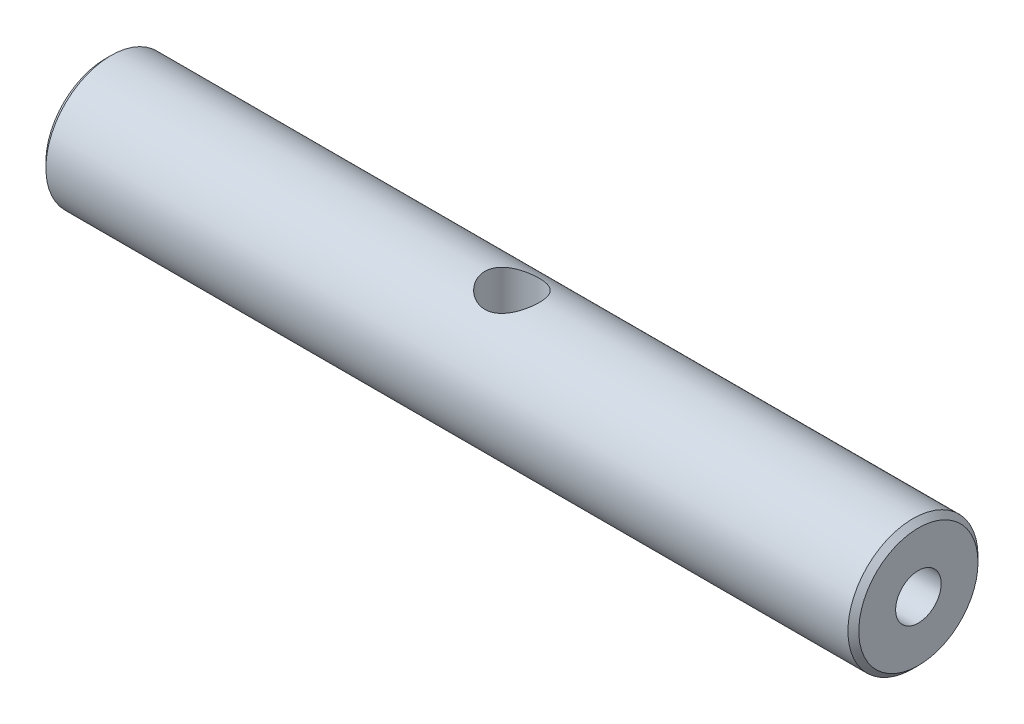
from build123d import *

# Parameters (mm, degrees)
SKETCH1_R             = 6
BOSS_EXTRUDE1_DEPTH   = 75
M5_TAPPED_HOLE1_D     = 4.2
M5_TAPPED_HOLE1_DEPTH = 12.4
M5_TAPPED_HOLE1_TIP   = 1.2618073
M5_TAPPED_HOLE2_D     = 4.2
M5_TAPPED_HOLE2_DEPTH = 12.4
M5_TAPPED_HOLE2_TIP   = 1.2618073
CHAMFER1_SIZE         = 0.5
SKETCH6_R             = 2.5
CUT_EXTRUDE1_DEPTH    = 17


with BuildPart() as part:
    # Sketch1 → Boss-Extrude1 (new body)
    with BuildSketch(Plane(origin=(0, 0, 0), x_dir=(0, 0, -1), z_dir=(1, 0, 0))):
        Circle(SKETCH1_R)
    extrude(amount=BOSS_EXTRUDE1_DEPTH)

    # M5 Tapped Hole1
    with Locations(Plane(origin=(75, 0, 0), x_dir=(0, 0, -1), z_dir=(1, 0, 0))):
        with Locations((0, 0)):
            Hole(M5_TAPPED_HOLE1_D / 2, depth=M5_TAPPED_HOLE1_DEPTH)
            with Locations((0, 0, -(M5_TAPPED_HOLE1_DEPTH + M5_TAPPED_HOLE1_TIP / 2))):  # 118° drill point
                Cone(0, M5_TAPPED_HOLE1_D / 2, M5_TAPPED_HOLE1_TIP, mode=Mode.SUBTRACT)

    # M5 Tapped Hole2
    with Locations(Plane.ZY):
        with Locations((0, 0)):
            Hole(M5_TAPPED_HOLE2_D / 2, depth=M5_TAPPED_HOLE2_DEPTH)
            with Locations((0, 0, -(M5_TAPPED_HOLE2_DEPTH + M5_TAPPED_HOLE2_TIP / 2))):  # 118° drill point
                Cone(0, M5_TAPPED_HOLE2_D / 2, M5_TAPPED_HOLE2_TIP, mode=Mode.SUBTRACT)

    # Chamfer1
    chamfer1_edges = [part.edges().sort_by_distance(p)[0] for p in [
        (0, 0, 6),
        (75, 0, 6),
    ]]
    chamfer(chamfer1_edges, length=CHAMFER1_SIZE)

    # Sketch6 → Cut-Extrude1 (cut, symmetric)
    with BuildSketch(Plane(origin=(0, 0, 0), x_dir=(1, 0, 0), z_dir=(0, 1, 0))):
        with Locations(Location((37.5, 0, 0), (0, 0, 270))):
            Circle(SKETCH6_R)
    extrude(amount=CUT_EXTRUDE1_DEPTH, both=True, mode=Mode.SUBTRACT)


solid = part.part
